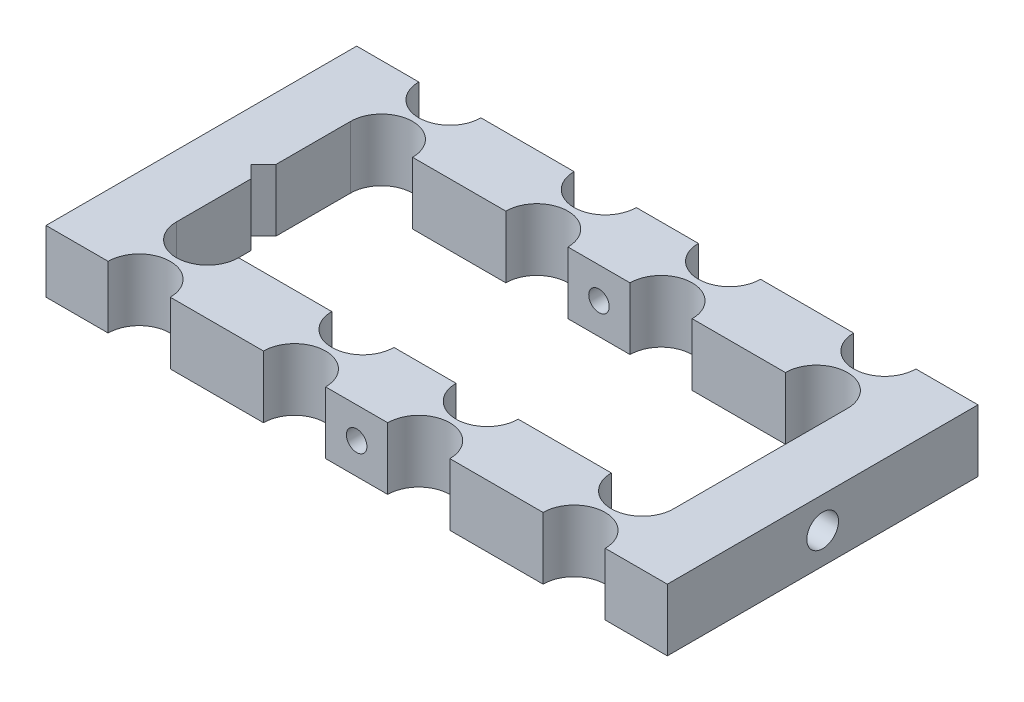
from build123d import *

# Parameters (mm, degrees)
BOSS_EXTRUDE1_DEPTH = 10
M4_TAPPED_HOLE1_D   = 3.3
CUT_EXTRUDE1_START  = -30
SKETCH4_R           = 2.55
CUT_EXTRUDE1_DEPTH  = 84
SCALE_FACTOR1_SCALE = 0.7


with BuildPart() as part:
    # Sketch1 → Boss-Extrude1 (new body)
    with BuildSketch(Plane(origin=(0, 0, 0), x_dir=(1, 0, 0), z_dir=(0, 1, 0))):
        with BuildLine():
            Line((-50, -25), (-40, -25))
            ThreePointArc((-40, -25), (-35, -20), (-30, -25))
            Line((-30, -25), (-15, -25))
            ThreePointArc((-15, -25), (-10, -20), (-5, -25))
            Line((-5, -25), (5, -25))
            ThreePointArc((5, -25), (10, -20), (15, -25))
            Line((15, -25), (30, -25))
            ThreePointArc((30, -25), (35, -20), (40, -25))
            Line((40, -25), (50, -25))
            Line((50, -25), (50, 25))
            Line((50, 25), (40, 25))
            ThreePointArc((40, 25), (35, 20), (30, 25))
            Line((30, 25), (15, 25))
            ThreePointArc((15, 25), (10, 20), (5, 25))
            Line((5, 25), (-5, 25))
            ThreePointArc((-5, 25), (-10, 20), (-15, 25))
            Line((-15, 25), (-30, 25))
            ThreePointArc((-30, 25), (-35, 20), (-40, 25))
            Line((-40, 25), (-50, 25))
            Line((-50, 25), (-50, -25))
        make_face()
        with BuildLine():
            Line((-40, 14), (-40, 2))
            Line((-40, 2), (-42, 0))
            Line((-42, 0), (-40, -2))
            Line((-40, -2), (-40, -14))
            ThreePointArc((-40, -14), (-35, -19), (-30, -14))
            Line((-30, -14), (-15, -14))
            ThreePointArc((-15, -14), (-10, -19), (-5, -14))
            Line((-5, -14), (5, -14))
            ThreePointArc((5, -14), (10, -19), (15, -14))
            Line((15, -14), (30, -14))
            ThreePointArc((30, -14), (35, -19), (40, -14))
            Line((40, -14), (40, 14))
            ThreePointArc((40, 14), (35, 19), (30, 14))
            Line((30, 14), (15, 14))
            ThreePointArc((15, 14), (10, 19), (5, 14))
            Line((5, 14), (0, 14))
            Line((0, 14), (-5, 14))
            ThreePointArc((-5, 14), (-10, 19), (-15, 14))
            Line((-15, 14), (-30, 14))
            ThreePointArc((-30, 14), (-35, 19), (-40, 14))
        make_face(mode=Mode.SUBTRACT)
    extrude(amount=BOSS_EXTRUDE1_DEPTH)

    # M4 Tapped Hole1 (through all)
    with Locations(Plane(origin=(0, 0, -25), x_dir=(-1, 0, 0), z_dir=(0, 0, -1))):
        with Locations((0, 5)):
            Hole(M4_TAPPED_HOLE1_D / 2)

    # Sketch4 → Cut-Extrude1 (cut)
    with BuildSketch(Plane.ZY.offset(50).offset(CUT_EXTRUDE1_START)):
        with Locations((0, 5)):
            Circle(SKETCH4_R)
    extrude(amount=-CUT_EXTRUDE1_DEPTH, mode=Mode.SUBTRACT)


with BuildPart() as part_1:
    # Scale factor1: scaled about (0, 0, 0)
    add(part.part.scale(SCALE_FACTOR1_SCALE))


solid = part_1.part
